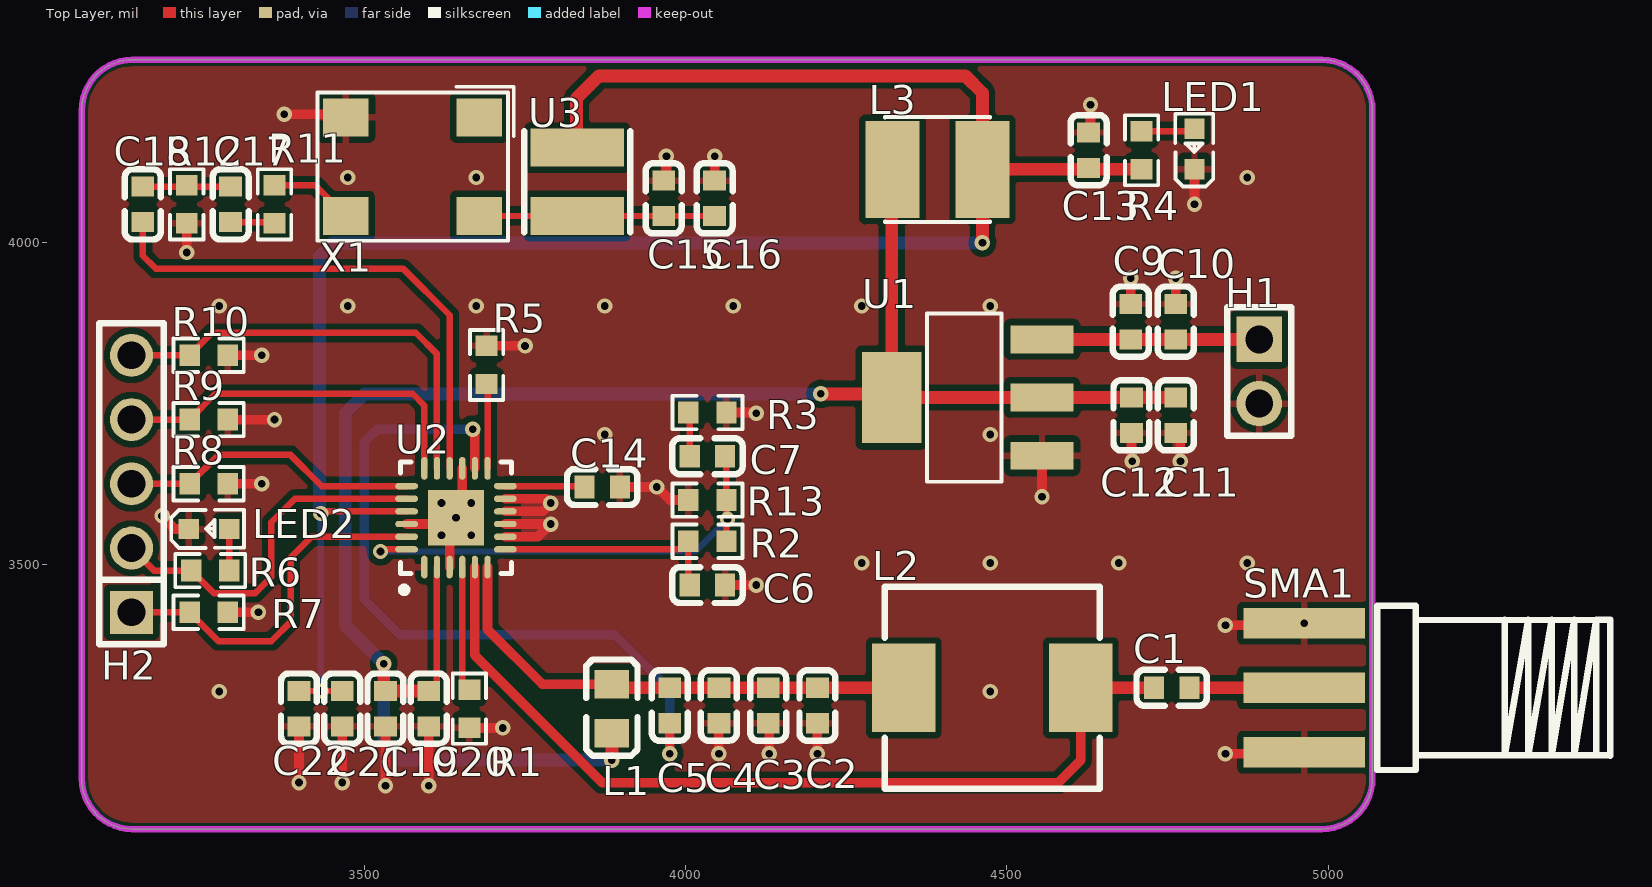
[diagram p0: Top Layer view]
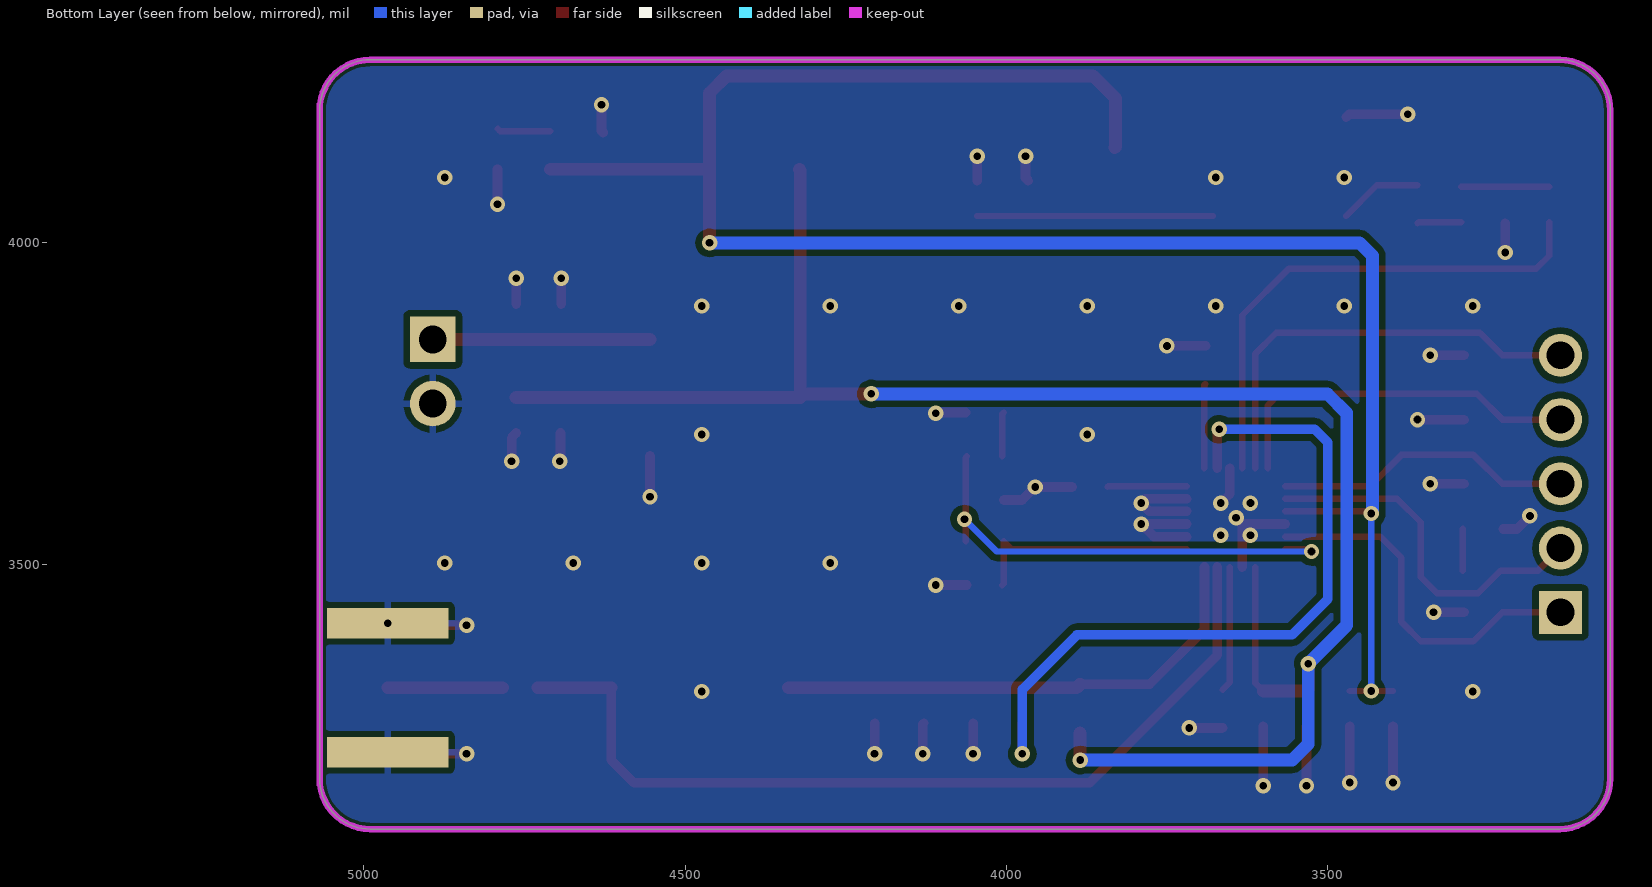
[diagram p1: Bottom Layer view, seen from below]
# Altium PCB MISC75048.pcbdoc
Units mil, origin at the board's own origin, x right, y up, seen from the top; angles counter-clockwise.
Board outline 2008.87 x 1197.37 mil, 2 copper layers (Top Layer, Bottom Layer), stack 62.206 mil thick; 46 components, 26 nets, 125 pads, 66 vias.

## Layer stack, top to bottom
Top Solder Mask Layer: solder mask 0.394, Dk 3.3
Top Layer: signal copper 1.379
Dielectric1: surface 59.449, FR4, Dk 4.5
Bottom Layer: signal copper 1.378
Bottom Solder Mask Layer: solder mask 0.394, Dk 3.3

## Board outline
3138.74,4285 ccw(c3138.74,4206.26) 3060,4206.26 3060,3166.38 ccw(c3138.74,3166.38) 3138.74,3087.64 4990.13,3087.64 ccw(c4990.13,3166.38) 5068.87,3166.38 5068.87,4206.26 ccw(c4990.13,4206.26) 4990.13,4285 3138.74,4285

## Design rules (kind name [scope] priority, off if disabled: settings)
BoardOutlineClearance copperThickness2oz_1 [All] p2 off: genericclearance=7.99 ignorepadtopadclearanceinfootprint=FALSE except(0: Arc-SplitContinuation Track-SplitContinuation SMDPad-SplitContinuation THPad-SplitContinuation Via-SplitContinuation Fill-SplitContinuation Region-SplitContinuation Poly-SplitContinuation Text-SplitContinuation Hole-SplitContinuation; 5.98: Arc-CutoutEdge Track-CutoutEdge SMDPad-CutoutEdge THPad-CutoutEdge Via-CutoutEdge Text-CutoutEdge; 6.9: Hole-OutlineEdge Hole-CutoutEdge; 10: Poly-OutlineEdge Poly-CutoutEdge; 11.81: Arc-OutlineEdge Track-OutlineEdge SMDPad-OutlineEdge THPad-OutlineEdge Via-OutlineEdge Fill-OutlineEdge Region-OutlineEdge Text-OutlineEdge Fill-CutoutEdge Region-CutoutEdge)
BoardOutlineClearance Plane_innerPlane_1 [All] p4 off: genericclearance=4.02 ignorepadtopadclearanceinfootprint=FALSE except(0: Arc-SplitContinuation Track-SplitContinuation SMDPad-SplitContinuation THPad-SplitContinuation Via-SplitContinuation Fill-SplitContinuation Region-SplitContinuation Poly-SplitContinuation Text-SplitContinuation Hole-SplitContinuation; 5.98: Arc-CutoutEdge Track-CutoutEdge SMDPad-CutoutEdge THPad-CutoutEdge Via-CutoutEdge Text-CutoutEdge; 6.9: Hole-OutlineEdge Hole-CutoutEdge; 10: Poly-OutlineEdge Poly-CutoutEdge; 11.81: Arc-OutlineEdge Track-OutlineEdge SMDPad-OutlineEdge THPad-OutlineEdge Via-OutlineEdge Fill-OutlineEdge Region-OutlineEdge Text-OutlineEdge Fill-CutoutEdge Region-CutoutEdge)
BoardOutlineClearance Copper_copperRegion_1 [All] p6 off: genericclearance=4.02 ignorepadtopadclearanceinfootprint=FALSE except(0: Arc-SplitContinuation Track-SplitContinuation SMDPad-SplitContinuation THPad-SplitContinuation Via-SplitContinuation Fill-SplitContinuation Region-SplitContinuation Poly-SplitContinuation Text-SplitContinuation Hole-SplitContinuation; 5.98: Arc-CutoutEdge Track-CutoutEdge SMDPad-CutoutEdge THPad-CutoutEdge Via-CutoutEdge Text-CutoutEdge; 6.9: Hole-OutlineEdge Hole-CutoutEdge; 10: Poly-OutlineEdge Poly-CutoutEdge; 11.81: Arc-OutlineEdge Track-OutlineEdge SMDPad-OutlineEdge THPad-OutlineEdge Via-OutlineEdge Fill-OutlineEdge Region-OutlineEdge Text-OutlineEdge Fill-CutoutEdge Region-CutoutEdge)
BoardOutlineClearance copperThickness1oz_1 [All] p8: genericclearance=4.02 ignorepadtopadclearanceinfootprint=FALSE except(0: Arc-SplitContinuation Track-SplitContinuation SMDPad-SplitContinuation THPad-SplitContinuation Via-SplitContinuation Fill-SplitContinuation Region-SplitContinuation Poly-SplitContinuation Text-SplitContinuation Hole-SplitContinuation; 5.98: Arc-CutoutEdge Track-CutoutEdge SMDPad-CutoutEdge THPad-CutoutEdge Via-CutoutEdge Text-CutoutEdge; 6.9: Hole-OutlineEdge Hole-CutoutEdge; 10: Poly-OutlineEdge Poly-CutoutEdge; 11.81: Arc-OutlineEdge Track-OutlineEdge SMDPad-OutlineEdge THPad-OutlineEdge Via-OutlineEdge Fill-OutlineEdge Region-OutlineEdge Text-OutlineEdge Fill-CutoutEdge Region-CutoutEdge)
Clearance copperThickness2oz [All] p1 off: gap=7.99 ignorepadtopadclearanceinfootprint=FALSE except(5.98: SMDPad-Track SMDPad-SMDPad THPad-Track SMDPad-THPad THPad-THPad Track-Via SMDPad-Via THPad-Via Via-Via Fill-SMDPad Region-SMDPad Fill-THPad Region-THPad Fill-Via Region-Via Fill-Fill Fill-Region Region-Region Arc-Track Arc-SMDPad Arc-THPad Arc-Via Fill-Arc Region-Arc Arc-Arc Text-Track SMDPad-Text Text-THPad Text-Via Fill-Text Region-Text Arc-Text Text-Text; 6.9: Hole-Track Hole-SMDPad Hole-THPad Hole-Via Fill-Hole Region-Hole Hole-Arc Hole-Text; 10: Poly-Track Poly-SMDPad Poly-THPad Poly-Via Poly-Fill Poly-Region Poly-Poly Poly-Arc Poly-Text Poly-Hole; 11.81: Fill-Track Region-Track)
Clearance Plane_innerPlane [All] p3 off: gap=4.02 ignorepadtopadclearanceinfootprint=FALSE except(5.98: SMDPad-Track SMDPad-SMDPad THPad-Track SMDPad-THPad THPad-THPad Track-Via SMDPad-Via THPad-Via Via-Via Fill-SMDPad Region-SMDPad Fill-THPad Region-THPad Fill-Via Region-Via Fill-Fill Fill-Region Region-Region Arc-Track Arc-SMDPad Arc-THPad Arc-Via Fill-Arc Region-Arc Arc-Arc Text-Track SMDPad-Text Text-THPad Text-Via Fill-Text Region-Text Arc-Text Text-Text; 6.9: Hole-Track Hole-SMDPad Hole-THPad Hole-Via Fill-Hole Region-Hole Hole-Arc Hole-Text; 10: Poly-Track Poly-SMDPad Poly-THPad Poly-Via Poly-Fill Poly-Region Poly-Poly Poly-Arc Poly-Text Poly-Hole; 11.81: Fill-Track Region-Track)
Clearance Copper_copperRegion [All] p5 off: gap=4.02 ignorepadtopadclearanceinfootprint=FALSE except(5.98: SMDPad-Track SMDPad-SMDPad THPad-Track SMDPad-THPad THPad-THPad Track-Via SMDPad-Via THPad-Via Via-Via Fill-SMDPad Region-SMDPad Fill-THPad Region-THPad Fill-Via Region-Via Fill-Fill Fill-Region Region-Region Arc-Track Arc-SMDPad Arc-THPad Arc-Via Fill-Arc Region-Arc Arc-Arc Text-Track SMDPad-Text Text-THPad Text-Via Fill-Text Region-Text Arc-Text Text-Text; 6.9: Hole-Track Hole-SMDPad Hole-THPad Hole-Via Fill-Hole Region-Hole Hole-Arc Hole-Text; 10: Poly-Track Poly-SMDPad Poly-THPad Poly-Via Poly-Fill Poly-Region Poly-Poly Poly-Arc Poly-Text Poly-Hole; 11.81: Fill-Track Region-Track)
Clearance copperThickness1oz [All] p7: gap=4.02 ignorepadtopadclearanceinfootprint=FALSE except(5.98: SMDPad-Track SMDPad-SMDPad THPad-Track SMDPad-THPad THPad-THPad Track-Via SMDPad-Via THPad-Via Via-Via Fill-SMDPad Region-SMDPad Fill-THPad Region-THPad Fill-Via Region-Via Fill-Fill Fill-Region Region-Region Arc-Track Arc-SMDPad Arc-THPad Arc-Via Fill-Arc Region-Arc Arc-Arc Text-Track SMDPad-Text Text-THPad Text-Via Fill-Text Region-Text Arc-Text Text-Text; 6.9: Hole-Track Hole-SMDPad Hole-THPad Hole-Via Fill-Hole Region-Hole Hole-Arc Hole-Text; 10: Poly-Track Poly-SMDPad Poly-THPad Poly-Via Poly-Fill Poly-Region Poly-Poly Poly-Arc Poly-Text Poly-Hole; 11.81: Fill-Track Region-Track)
DiffPairsRouting differentialPair [All] p1: maxlimit=6 minlimit=6 mostfreqgap=6 toplayer_minwidth=5 toplayer_prefwidth=10 toplayer_maxwidth=100 toplayer_mingap=6 toplayer_prefgap=6 toplayer_maxgap=6 bottomlayer_minwidth=5 bottomlayer_prefwidth=10 bottomlayer_maxwidth=100 bottomlayer_mingap=6 bottomlayer_prefgap=6 bottomlayer_maxgap=6 maxuncoupledlength=10
HoleToHoleClearance otherClearance [All] p1: gap=11.81 allowstackedmicrovias=TRUE
Length netLength [All] p1: minlimit=0 maxlimit=0
PasteMaskExpansion pasteMaskExpansion [All] p1: expansion=0
PlaneConnect innerPlane [All] p1: planeconnectstyle=Relief reliefexpansion=20 reliefentries=4 reliefconductorwidth=10 reliefairgap=10
PolygonConnect copperRegion [All] p1: connectstyle=Relief reliefconductorwidth=10 reliefentries=4 polygonreliefangle="90 Angle" airgapwidth=10 via.connectstyle=Relief via.reliefconductorwidth=10 via.reliefentries=4 via.polygonreliefangle="90 Angle" via.airgapwidth=10
RoutingVias viaSize [All] p1: holewidth=12.01 width=24.02 viastyle="Through Hole" minholewidth=11.81 minwidth=19.68 maxholewidth=248.03 maxwidth=393.7
SolderMaskExpansion solderMaskExpansion [IsVia] p1: expansion=-1000 istentingtop=TRUE
SolderMaskExpansion solderMaskExpansion [All] p2: expansion=2 istentingtop=FALSE
Width copperThickness2oz_2 [All] p1 off: maxlimit=100 minlimit=8 preferedwidth=10
Width copperThickness1oz_2 [All] p2: maxlimit=100 minlimit=5 preferedwidth=10

## Components (designator, comment, footprint, x,y, rotation, side; value= is the part's Value field where it differs from the comment)
C1 "10pF" C0603 4756.35,3307.56 r0 top
C2 "10pF" C0603 4205,3280 r90 top
C3 "10pF" C0603 4128.33,3280 r90 top
C4 "10pF" C0603 4051.67,3280 r90 top
C5 "10nF" C0603 3975,3280 r90 top
C6 "33pF" C0603 4033.76,3467.45 r180 top
C7 "150pF" C0603 4033.76,3667.86 r0 top
C9 "0.1uF" C0603 4692.65,3877.34 r270 top
C10 "47uF" C0603 4762.65,3877.34 r270 top
C11 "0.1uF" C0603 4762.87,3731.67 r90 top
C12 "10uF" C0603 4693.74,3731.67 r90 top
C13 "10uF" C0603 4627.08,4144.23 r270 top
C14 "1nF" C0603 3870,3620 r180 top
C15 "100pF" C0603 3965.63,4069.41 r270 top
C16 "0.1uF" C0603 4045,4069.41 r270 top
C17 "1nF" C0603 3291.67,4060 r90 top
C18 "1nF" C0603 3155,4060 r270 top
C19 "100pF" C0603 3532.68,3275 r90 top
C20 "0.1uF" C0603 3599.99,3275 r90 top
C21 "100pF" C0603 3465.38,3275 r90 top
C22 "0.1uF" C0603 3398.07,3275 r90 top
H1 "" HDR-TH_2P-P2.54-V-M-1 4892.65,3799.78 r270 top
H2 "" HDR-TH_5P-P2.54-V-M 3137.47,3625 r90 top
L1 "100nH" L0805 3885,3275 r270 top
L2 "15uH" IND-SMD_L8.5-W8.0-LS9.5_ZEYH0850-15UH 4477.22,3307.56 r0 top
L3 "100uH" IND-SMD_L4.0-W4.0_SWPA4018S 4391.81,4114.23 r180 top
LED1 "" LED_0603 4791.51,4148.18 r90 top
LED2 "" LED_0603 3260,3555 r0 top
R1 "51R" R0603 3663.34,3275 r90 top
R2 "0KR" R0603 4033.76,3535.57 r180 top
R3 "13KR" R0603 4033.76,3735.99 r0 top
R4 "51R" R0603 4709.55,4144.23 r270 top
R5 "4.7KR" R0603 3690,3810 r270 top
R6 "1KR" R0603 3260,3490 r180 top
R7 "10KR" R0603 3257.47,3425 r0 top
R8 "10KR" R0603 3257.47,3625 r0 top
R9 "10KR" R0603 3257.47,3725 r0 top
R10 "10KR" R0603 3257.47,3825 r0 top
R11 "0R" R0603 3360,4060 r90 top
R12 "51R" R0603 3223.33,4060 r270 top
R13 "NC" R0603 4033.76,3599.74 r180 top
SMA1 "SMA" SMA-SMD_BWSMA-KE-P001 4962.57,3307.56 r0 top
U1 "AMS1117-3.3" SOT-223-3_L6.5-W3.4-P2.30-LS7.0-BR 4437.65,3759.23 r0 top
U2 "ADF4360-0BCPZ" LFCSP-24_L4.0-W4.0-P0.50-BL-EP2.3 3642.36,3572.23 r0 top
U3 "10uH" IND-SMD_L4.0-W4.0_LVF404015 3831.14,4095 r270 top
X1 "16MHz" OSC-SMD_4P-L7.0-W5.0-BL 3575,4118.62 r180 top

## Footprints (in the part's own frame and the unit in brackets; to place one, negate y for a bottom-side part, rotate by r counter-clockwise, add the part's x,y. Pads: shape width x height; smd on the part's side, far side on the other; paste and mask are expansions set on the pad)
C0603 [mm]
  rect 0.8x0.9 smd: 1(-0.7,0) 2(0.7,0)
  silkscreen extent -1.39,-0.71 1.39,0.71
HDR-TH_2P-P2.54-V-M-1 [mm]
  rect 1.8x1.8 hole 1.1: 1(-1.27,0)
  round 1.8 hole 1.1: 2(1.27,0)
  silkscreen extent -2.54,-1.27 2.54,1.27
HDR-TH_5P-P2.54-V-M [mm]
  rect 1.7x1.7 hole 1.1: 1(-5.08,0)
  round 1.7 hole 1.1: 2(-2.54,0) 3(0,0) 4(2.54,0) 5(5.08,0)
  silkscreen extent -6.35,-1.27 6.35,1.27
IND-SMD_L4.0-W4.0_LVF404015 [mm]
  rect 1.5x3.7 smd: 1(-1.35,0) 2(1.35,0)
  silkscreen extent -2,-2.1 2,2.1
IND-SMD_L4.0-W4.0_SWPA4018S [mil]
  rect 83.62x150.39 smd: 1(70,0) 2(-70,0)
  silkscreen extent -82,-82 82,82
IND-SMD_L8.5-W8.0-LS9.5_ZEYH0850-15UH [mm]
  rect 2.5x3.5 smd: 1(-3.5,0) 2(3.5,0)
  silkscreen extent -4.25,-4 4.25,4
L0805 [mil]
  rect 44.59x54.21 smd paste-3937.01 mask+2: 1(-38.04,0) 2(38.04,0)
  silkscreen extent -77,-40 73,40
LED_0603 [mil]
  rect 31.5x31.5 smd paste+0 mask+2: 1(-33.5,-0.4) 2(29.5,-0.2)
  silkscreen extent -61,-30 53,30
LFCSP-24_L4.0-W4.0-P0.50-BL-EP2.3 [mm]
  oval 0.25x0.9 smd paste-100 mask+0.05: 1(-1.25,-1.951) 2(-0.75,-1.951) 3(-0.25,-1.951) 4(0.25,-1.951) 5(0.75,-1.951) 6(1.25,-1.951) 13(1.25,1.951) 14(0.75,1.951) 15(0.25,1.951) 16(-0.25,1.951) 17(-0.75,1.951) 18(-1.25,1.951)
  oval 0.9x0.25 smd paste-100 mask+0.05: 7(1.951,-1.25) 8(1.951,-0.75) 9(1.951,-0.25) 10(1.951,0.25) 11(1.951,0.75) 12(1.951,1.25) 19(-1.951,1.25) 20(-1.951,0.75) 21(-1.951,0.25) 22(-1.951,-0.25) 23(-1.951,-0.75) 24(-1.951,-1.25)
  rect 2.2x2.2 smd paste-100 mask+0.05: 25(0,0)
  silkscreen extent -2.2,-2.98 2.2,2.2
OSC-SMD_4P-L7.0-W5.0-BL [mm]
  rect 1.8x1.5 smd: 1(-2.64,-1.95) 2(2.64,-1.95) 3(2.64,1.95) 4(-2.64,1.95)
  silkscreen extent -4,-3.16 3.77,2.93
R0603 [mil]
  rect 31.75x34.02 smd paste-3937.01 mask+2: 1(-29.66,0) 2(29.66,0)
  silkscreen extent -55,-26 55,26
SMA-SMD_BWSMA-KE-P001 [mm]
  rect 4.8x1.2 smd: 1(0,-2.55) 2(0,2.55) 5(0,0)
  rect 4.8x1.2 smd far side: 3(0,2.55) 4(0,-2.55)
  Board Outline Layer lines w0.254: 2.7,-3.3 2.7,3.3
  silkscreen extent 2.89,-3.25 12.1,3.25
SOT-223-3_L6.5-W3.4-P2.30-LS7.0-BR [mm]
  rect 2.5x1.1 smd: 1(2.97,-2.3) 2(2.97,0) 3(2.97,2.3)
  rect 2.34x3.6 smd: 4(-2.97,0)
  silkscreen extent -1.57,-3.33 1.37,3.33

## Via types
v1: diameter 24.02, hole 12, Top Layer to Bottom Layer, 66 vias

## Nets (pads, with @x,y where several pads share a name; then routed paths per layer and width w, separated by ;. In a path a pad name is that pad's centre, name@x,y a point inside that pad or via, vN(x,y) a via of type N, cw(c..) or ccw(c..) an arc to the next point about the centre after c; other vN are vias at no path point)
$1N308: C1.2 SMA1.5 | length 178.7
  Top Layer w20: C1.2 SMA1.5
$1N1101: C9.2 C10.2 H1.1 U1.3 | length 338.1
  Top Layer w20: U1.3 C9.2 C10.2 H1.1
$1N1480: LED1.2 R4.1 | length 83.7
  Top Layer w10: R4.1 4787.92,4173.89 LED1.2
$1N1873: R5.2 U2.13 | length 132
  Top Layer w10: R5.2 3691.57,3778.77 U2.13
$1N1955: C14.2 U2.12 | length 123.9
  Top Layer w10: U2.12 3841.01,3621.43 C14.2
$1N2023: LED2.2 R6.1 | length 64.9
  Top Layer w10: LED2.2 3289.66,3554.64 R6.1
$1N2408: C15.2 C16.2 U3.2 X1.4 | length 366.1
  Top Layer w10: X1.4 U3.2 C15.2 C16.2
$1N2649: R11.2 X1.3 | length 130.9
  Top Layer w10: R11.2 3423.25,4089.66 X1.3
$1N2699: C17.1 R11.1 | length 69.2
  Top Layer w10: C17.1 3357.9,4032.44 R11.1
$1N2725: C17.2 C18.1 R12.1 | length 136.7
  Top Layer w10: C18.1 C17.2
$1N3994: C7.1 R3.1 | length 69
  Top Layer w10: R3.1 4006.2,3733.89 C7.1
AVDD: C11.2 C12.2 C19.2 C20.2 L1.2 L3.1 U1.2 U1.4 U2.2 | length 2919.4
  Top Layer w10: C20.2 3612.83,3315.4 U2.2
  Top Layer w20: v1(3530,3345) 3530,3305.24 C19.2 C20.2 ; v1(3885,3195) L1.2 ; v1(4210,3765) 4314.95,3765 U1.4 ; L3.1 4320.72,4113.14 U1.4 ; C11.2 C12.2 U1.2 U1.4
  Bottom Layer w20: v1(3885,3195) 3555,3195 3530,3220 v1(3530,3345) 3470,3405 3470,3735 3500,3765 v1(4210,3765)
CE: H2.1 R7.1 U2.23 | length 572.7
  Top Layer w10: H2.1 R7.1 3272.81,3380 3355,3380 3385,3410 3385,3510 3417.69,3542.69 U2.23
CLK: H2.5 R10.1 U2.17 | length 681.6
  Top Layer w10: H2.5 R10.1 3262.81,3860 3580,3860 3612.83,3827.17 U2.17
CN: C5.1 U2.14 | length 1166.5
  Top Layer w15: v1(3668.57,3710) 3671.91,3706.67 U2.14 ; v1(3975,3205) C5.1
  Bottom Layer w15: v1@3670,3710 3520,3710 3499.51,3689.51 3499.51,3445.49 3555,3390 3890,3390 3975,3305 v1(3975,3205)
CP: C7.2 R2.1 R13.1 U2.24 | length 735.9
  Top Layer w10: v1(3525,3519.7) 3528.33,3523.03 U2.24 ; C7.2 4063.42,3665.76 R13.1 R2.1
  Bottom Layer w10: v1(3525,3519.7) 4014.7,3519.7 v1(4065,3570)
DATA: H2.4 R9.1 U2.18 | length 577.6
  Top Layer w10: H2.4 R9.1 3267.81,3765 3575,3765 3593.17,3746.83 U2.18
DVDD: C13.2 C21.2 C22.2 L3.2 R4.2 U2.21 U3.1 | length 3142.3
  Top Layer w10: C22.2 v1(3431.99,3302.56) C21.2 ; v1(3431.99,3578.78) 3435.28,3582.07 U2.21 ; C13.2@4624.98,4114.57 C13.2 C13.2@4629.18,4114.57
  Top Layer w20: U3.1 3830,4149.29 3830,4225 3865,4260 4435,4260 4461.81,4233.19 L3.2 ; v1(4461.81,4000) L3.2 ; R4.2 4629.18,4114.57 4624.98,4114.57 4462.15,4114.57 L3.2
  Bottom Layer w10: v1(3431.99,3302.56) v1(3431.99,3578.78)
  Bottom Layer w20: v1(3431.99,3578.78) 3430,3580.77 3430,3980 3450,4000 v1(4461.81,4000)
GND: C2.1 C3.1 C4.1 C6.1 C9.1 C10.1 C11.1 C12.1 C13.1 C14.1 C15.1 C16.1 C19.1 C20.1 C21.1 C22.1 H1.2 LED1.1 LED2.1 R1.1 R3.2 R5.1 R7.2 R8.2 R9.2 R10.2 R12.2 R13.2 SMA1.1 SMA1.2 SMA1.3 SMA1.4 U1.1 U2.1 U2.3 U2.8 U2.9 U2.10 U2.11 U2.15 U2.22 U2.25 X1.2 | length 2411.9
  Top Layer w15: v1(3185,3575) 3205.4,3554.6 LED2.1 ; v1(3223.33,3985) R12.2 ; R7.2 v1(3335,3425) ; R8.2 v1(3340,3625) ; R9.2 v1(3360,3725) ; R10.2 v1(3340,3825) ; v1(3375,4200) 3466.45,4200 X1.2 ; v1(3398.07,3160) C22.1 ; v1(3465.38,3160) C21.1 ; v1(3532.68,3155) C19.1 ; U2.22 3632.53,3562.39 v1(3642.37,3572.23) ; v1(3600,3155) C20.1 ; U2.3 U2.25@3632.52,3562.38 ; U2.15 3652.21,3608.79 v1(3666,3595) ; R1.1 3663.68,3245 v1(3715,3245) ; R5.1 v1(3750,3839.66) ; U2.8 3770.3,3542.69 v1(3790,3562.39) U2.9 ; U2.10 3777.07,3582.07 v1(3790,3595) 3783.23,3601.77 U2.11 ; C14.1 v1(3955,3620) 3975.26,3599.74 R13.2 ; C15.1 3970,4101.34 v1(3970,4135) ; C16.1 v1(4045,4135) ; v1(4051.67,3205) C4.1 ; C6.1 v1(4110,3467.45) ; R3.2 4109.01,3735.99 v1(4110,3735) ; C3.1 4130,3250.77 v1(4130,3205) ; v1(4205,3205) C2.1 ; v1(4554.58,3605) U1.1 ; C13.1 4630,4174.72 v1(4630,4215) ; C9.1 v1(4692.65,3945) ; C12.1 4693.74,3661.26 v1(4695,3660) ; C10.1 v1(4762.65,3945) ; C11.1 4770,3696.98 v1(4770,3660) ; v1(4791.91,4060) LED1.1 ; v1(4840,3205) 4960.41,3205 SMA1.1 ; v1(4840,3405) 4959.63,3405 v1(4962.58,3407.95)
  other v1: 3274.1,3301.74 4474.1,3301.74 4274.1,3501.74 4474.1,3501.74 4674.1,3501.74 4874.1,3501.74 3620,3545 3666,3545 3620,3595 3874.1,3701.74 4474.1,3701.74 3274.1,3901.74 3474.1,3901.74 3674.1,3901.74 3874.1,3901.74 4074.1,3901.74 4274.1,3901.74 4474.1,3901.74 3474.1,4101.73 3674.1,4101.73 4874.1,4101.73
LE: H2.3 R8.1 U2.19 | length 466.9
  Top Layer w10: H2.3 R8.1 3272.81,3670 3385,3670 3433.57,3621.43 U2.19
MUXOUT: H2.2 R6.2 U2.20 | length 567.7
  Top Layer w10: H2.2 3172.47,3490 R6.2 3265.34,3455 3330,3455 3355,3480 3355,3565 3391.77,3601.77 U2.20
RA: R1.2 U2.4 | length 195.4
  Top Layer w10: U2.4 3652.21,3315.8 R1.2
RB: C1.1 L2.2 U2.5 | length 1403.3
  Top Layer w15: U2.5 3671.91,3358.09 3870,3160 4580,3160 4615.01,3195.01 L2.2
  Top Layer w20: L2.2 C1.1
REFIN: C18.2 U2.16 | length 806.7
  Top Layer w10: C18.2 3155,3980 3175,3960 3560,3960 3632.53,3887.47 U2.16
VTURN: C6.2 R2.2 U2.7 | length 359.1
  Top Layer w10: U2.7 3991.56,3523.03 R2.2 4004.1,3469.55 C6.2
VVCO: C2.2 C3.2 C4.2 C5.2 L1.1 L2.1 U2.6 | length 782.5
  Top Layer w15: U2.6 3691.57,3398.43 3776.96,3313.04 L1.1
  Top Layer w20: L1.1 3890.48,3307.56 C5.2 C4.2 C3.2 C2.2 L2.1
pads on no net: X1.1

## Polygon pours and split planes (outlines as drawn)
GND on Top Layer (solid, remove dead copper, pour order 0): 3000,4475 3000,3015 5220,3015 5220,4475
GND on Bottom Layer (solid, remove dead copper, pour order 2): 3015,4390 3015,3000 5190,3000 5190,4390

## Keep-outs
Board Outline Layer:
  the board outline again, w10